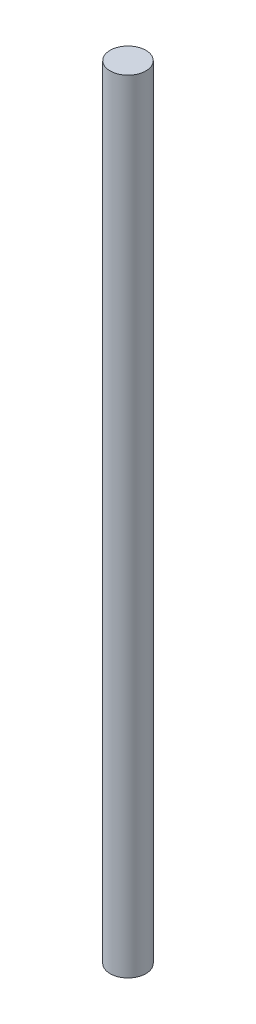
SolidWorks part; units mm, degrees
material "Cu"
ref_plane "Front Plane" through (0, 0, 0) normal (0, 0, 1) x (1, 0, 0)
ref_plane "Top Plane" through (0, 0, 0) normal (0, 1, 0) x (1, 0, 0)
ref_plane "Right Plane" through (0, 0, 0) normal (1, 0, 0) x (0, 0, -1)
sketch "Sketch1" plane through (0, 0, 0) normal (0, 1, 0) x (1, 0, 0)
  circle A0 centre (0, 0) radius 0.8
  dimension "D1" = 1.6
extrude "Boss-Extrude1" add sketch "Sketch1" along normal blind 35
